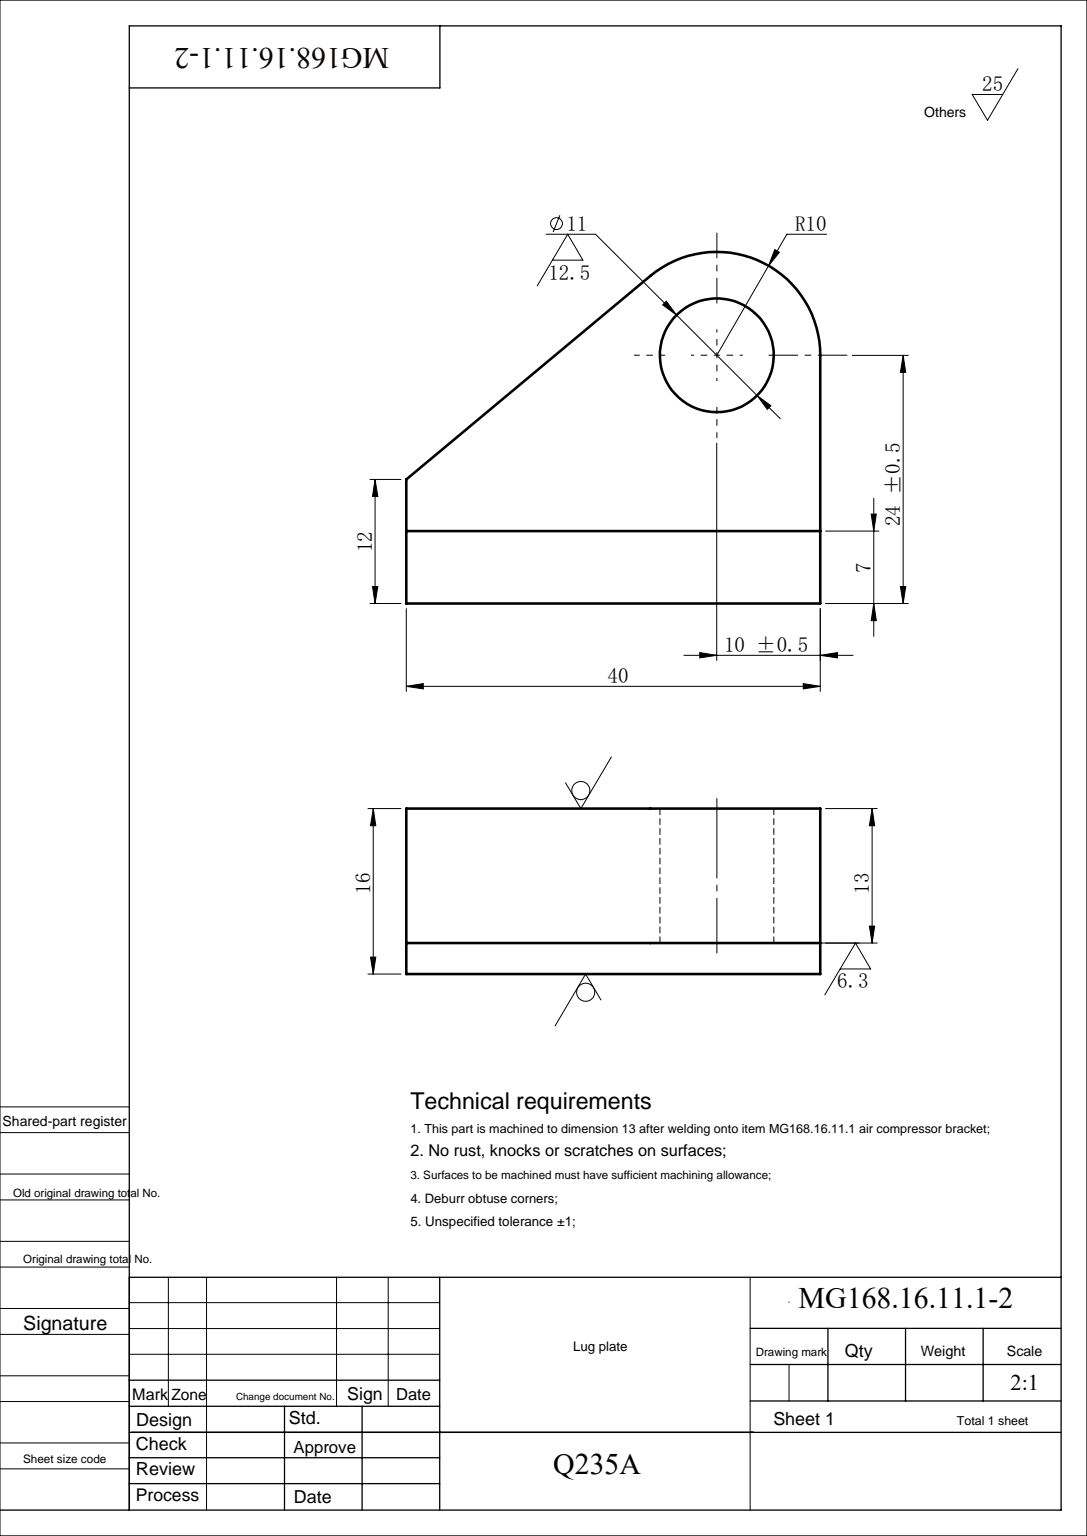
from build123d import *

# Parameters (mm, degrees)
SKETCH1_R           = 5.5
BOSS_EXTRUDE1_DEPTH = 6.5
SKETCH2_W           = 40
SKETCH2_H           = 7
BOSS_EXTRUDE2_DEPTH = 3


with BuildPart() as part:
    # Sketch1 → Boss-Extrude1 (new, symmetric)
    with BuildSketch(Plane(origin=(0, 0, 0), x_dir=(1, 0, 0), z_dir=(0, 1, 0))):
        with BuildLine():
            Line((40, 12), (16.405124482, 31.679477871))
            ThreePointArc((16.405124482, 31.679477871), (5.760380018, 33.056799788), (0, 24))
            Line((0, 24), (0, 0))
            Line((0, 0), (40, 0))
            Line((40, 0), (40, 12))
        make_face()
        with Locations(Location((10, 24, 0), (0, 0, 90))):
            Circle(SKETCH1_R, mode=Mode.SUBTRACT)
    extrude(amount=BOSS_EXTRUDE1_DEPTH, both=True)

    # Sketch2 → Boss-Extrude2 (add)
    with BuildSketch(Plane(origin=(0, -6.5, 0), x_dir=(1, 0, 0), z_dir=(0, 1, 0))):
        with Locations((20, 3.5)):
            Rectangle(SKETCH2_W, SKETCH2_H)
    extrude(amount=-BOSS_EXTRUDE2_DEPTH)


solid = part.part
